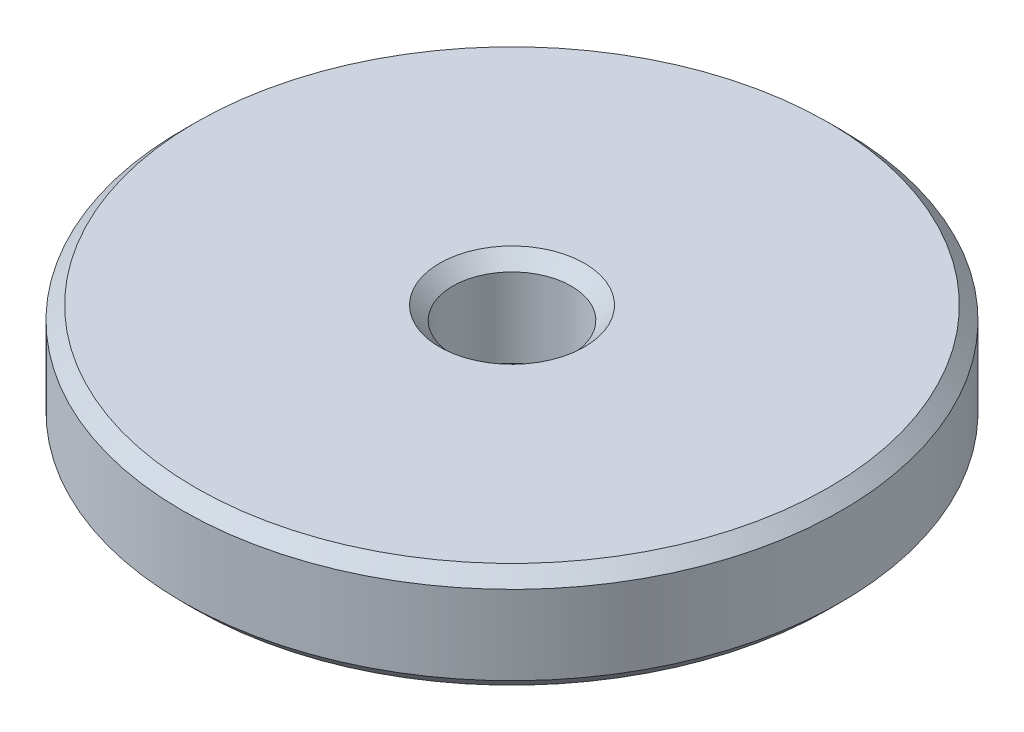
SolidWorks part; units mm, degrees
ref_plane "前视基准面" through (0, 0, 0) normal (0, 0, 1) x (1, 0, 0)
ref_plane "上视基准面" through (0, 0, 0) normal (0, 1, 0) x (1, 0, 0)
ref_plane "右视基准面" through (0, 0, 0) normal (1, 0, 0) x (0, 0, -1)
sketch "草图1" plane through (0, 0, 0) normal (0, 0, 1) x (1, 0, 0)
  line L0 (24, 8) -> (5.5, 8)
  line L1 (5.5, 8) -> (4.5, 7)
  line L2 (4.5, 7) -> (4.5, 1)
  line L3 (4.5, 1) -> (5.5, 0)
  line L4 (5.5, 0) -> (24, 0)
  line L5 (24, 0) -> (25, 1)
  line L6 (25, 1) -> (25, 7)
  line L7 (25, 7) -> (24, 8)
  line L8 (0, 8) -> (0, 0) construction
revolve "旋转1" add sketch "草图1" angle 360 about L8
